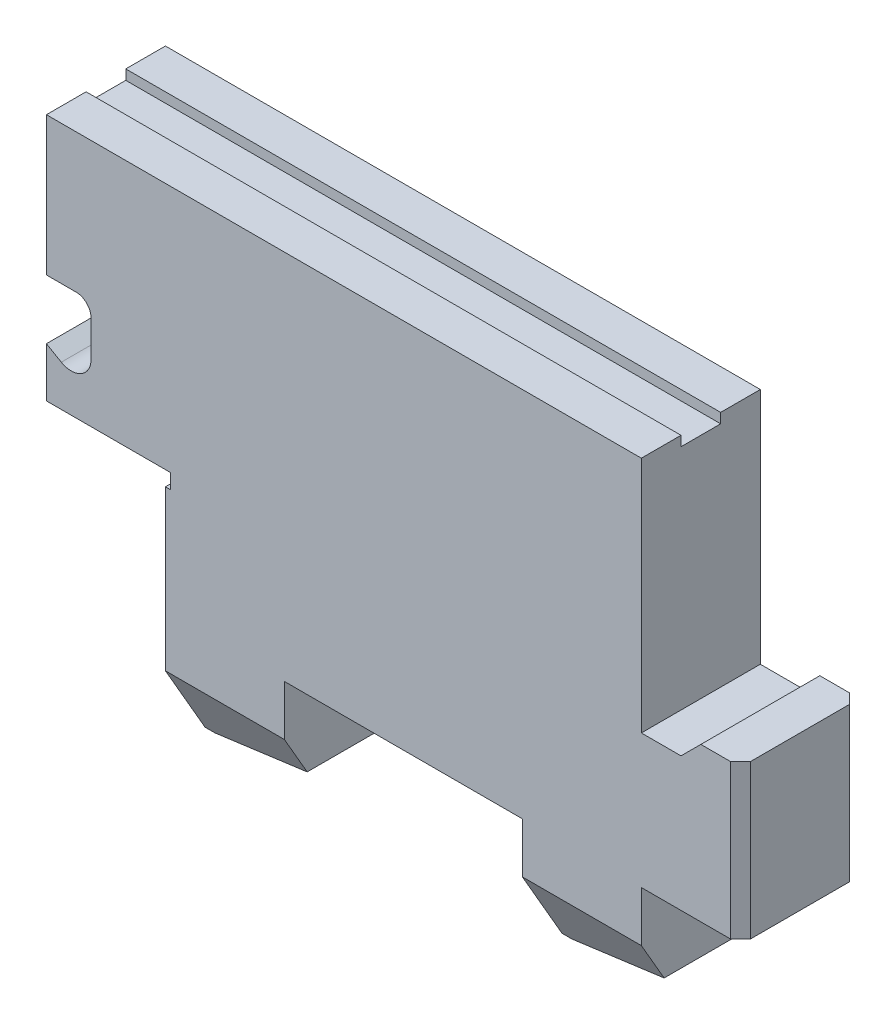
from build123d import *

# Parameters (mm, degrees)
EXTRUDE_1_DEPTH     = 6
CUT_EXTRUDE_1_DEPTH = 64.442887702
SKETCH_3_W          = 60
SKETCH_3_H          = 4
CUT_EXTRUDE_2_DEPTH = 1
CHAMFER_1_SIZE      = 1


with BuildPart() as part:
    # 草图1 → 凸台-拉伸1 (new, symmetric)
    with BuildSketch(Plane.XY):
        with BuildLine():
            Line((0, 0), (0, 5))
            Line((0, 5), (1.5, 4.133974596))
            ThreePointArc((1.5, 4.133974596), (3.5, 4.133974596), (4.5, 5.866025404))
            Line((4.5, 5.866025404), (4.5, 9.5))
            ThreePointArc((4.5, 9.5), (4.060660172, 10.560660172), (3, 11))
            Line((3, 11), (0, 11))
            Line((0, 11), (0, 25))
            Line((0, 25), (60, 25))
            Line((60, 25), (60, 1))
            Line((60, 1), (64, 1))
            Line((64, 1), (66, 3))
            Line((66, 3), (70, 3))
            Line((70, 3), (70, -12.5))
            Line((70, -12.5), (60, -12.5))
            Line((60, -12.5), (60, -21.552558883))
            Line((60, -21.552558883), (49, -24.5))
            Line((49, -24.5), (48, -24.5))
            Line((48, -24.5), (48, -12.5))
            Line((48, -12.5), (24, -12.5))
            Line((24, -12.5), (24, -21.552558883))
            Line((24, -21.552558883), (13, -24.5))
            Line((13, -24.5), (12, -24.5))
            Line((12, -24.5), (12, -1.5))
            Line((12, -1.5), (12.5, -1.5))
            Line((12.5, -1.5), (12.5, 0))
            Line((12.5, 0), (0, 0))
        make_face()
    extrude(amount=EXTRUDE_1_DEPTH, both=True)

    # 草图2 → 切除-拉伸1 (cut, through all)
    with BuildSketch(Plane.ZY.offset(-12)):
        Polygon((6, -17.57179677), (6, -29.5), (-6, -29.5), (-6, -17.57179677), (-2, -24.5), (2, -24.5), align=None)
    extrude(amount=-CUT_EXTRUDE_1_DEPTH, mode=Mode.SUBTRACT)

    # 草图3 → 切除-拉伸2 (cut)
    with BuildSketch(Plane(origin=(0, 25, 0), x_dir=(1, 0, 0), z_dir=(0, 1, 0))):
        with Locations((30, 0)):
            Rectangle(SKETCH_3_W, SKETCH_3_H)
    extrude(amount=-CUT_EXTRUDE_2_DEPTH, mode=Mode.SUBTRACT)

    # 倒角1
    chamfer_1_edges = [part.edges().sort_by_distance(p)[0] for p in [
        (70, -4.75, -6),
        (70, -4.75, 6),
    ]]
    chamfer(chamfer_1_edges, length=CHAMFER_1_SIZE)


solid = part.part
